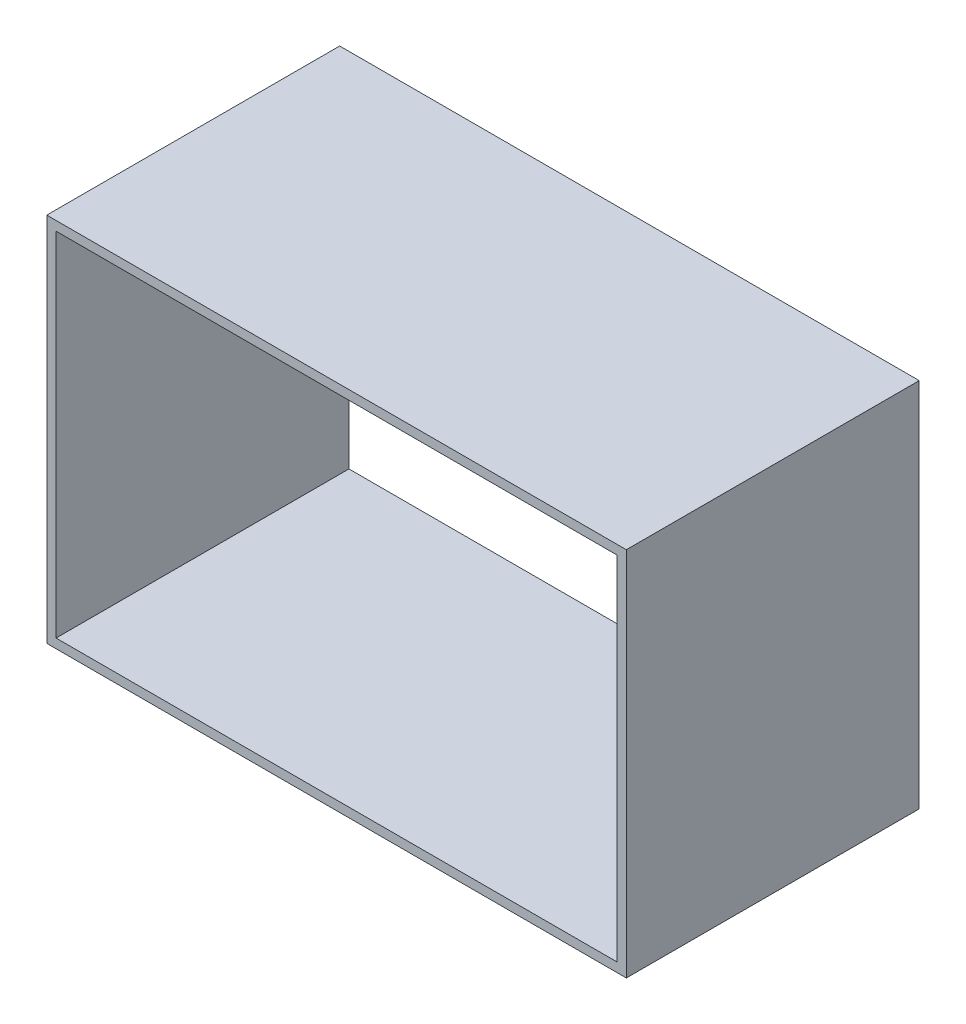
SolidWorks part; units mm, degrees
ref_plane "Front Plane" through (0, 0, 0) normal (0, 0, 1) x (1, 0, 0)
ref_plane "Top Plane" through (0, 0, 0) normal (0, 1, 0) x (1, 0, 0)
ref_plane "Right Plane" through (0, 0, 0) normal (1, 0, 0) x (0, 0, -1)
other "Configuration Table"
sketch "Sketch1" plane through (0, 0, 0) normal (0, 0, 1) x (1, 0, 0)
  line L1 (0, 0) -> (500, 0)
  line L2 (0, 0) -> (0, 320)
  line L3 (0, 320) -> (500, 320)
  line L4 (500, 0) -> (500, 320)
  line L5 (8, 312) -> (492, 312)
  line L6 (8, 312) -> (8, 8)
  line L7 (8, 8) -> (492, 8)
  line L8 (492, 312) -> (492, 8)
  dimension "D1" = 500
  dimension "D2" = 320
  dimension "D3" = 8
  dimension "D4" = 8
  dimension "D5" = 8
  dimension "D6" = 8
extrude "Boss-Extrude1" add sketch "Sketch1" along normal blind 252.7
